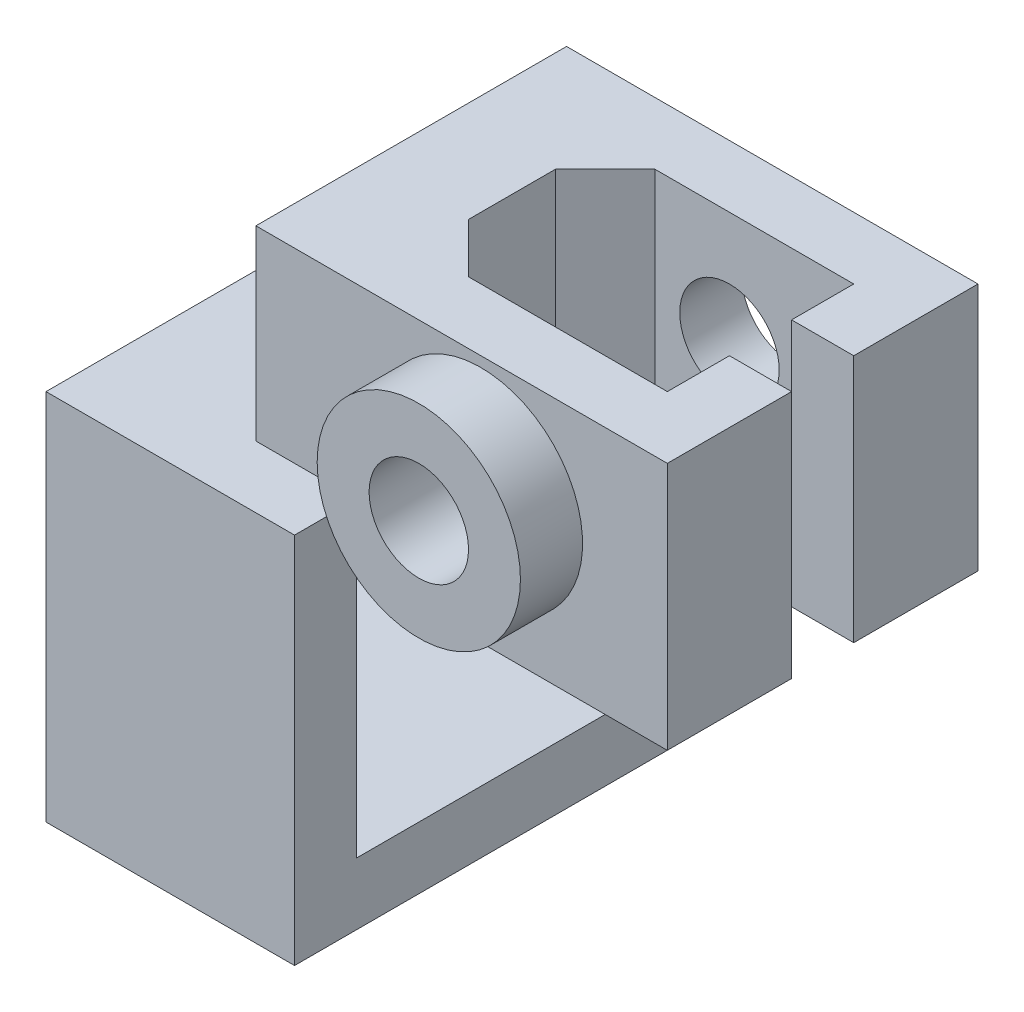
SolidWorks part; units mm, degrees
ref_plane "Front Plane" through (0, 0, 0) normal (0, 0, 1) x (1, 0, 0)
ref_plane "Top Plane" through (0, 0, 0) normal (0, 1, 0) x (1, 0, 0)
ref_plane "Right Plane" through (0, 0, 0) normal (1, 0, 0) x (0, 0, -1)
other "Configuration Table"
sketch "Sketch1" plane through (0, 0, 0) normal (0, 1, 0) x (1, 0, 0)
  line L1 (-20, 25) -> (20, 25)
  line L2 (-20, 25) -> (-20, -25)
  line L3 (-20, -25) -> (20, -25)
  line L4 (20, 25) -> (20, -25)
  line L5 (-20, 25) -> (20, -25) construction
  line L6 (-20, -25) -> (20, 25) construction
  point P0 (0, 0)
  dimension "D1" = 50
  dimension "D2" = 40
extrude "Boss-Extrude1" add sketch "Sketch1" along normal blind 10
sketch "Sketch2" plane through (0, 10, 0) normal (0, 1, 0) x (1, 0, 0)
  line L0 (28, -15) -> (60, -15)
  line L1 (20, -25) -> (20, 25) construction
  line L2 (60, -15) -> (60, -5)
  line L3 (60, -5) -> (70, -5)
  line L4 (70, -5) -> (70, -25)
  line L5 (70, -25) -> (20, -25)
  line L6 (20, -25) -> (20, -15)
  line L7 (20, 25) -> (70, 25)
  line L8 (70, 25) -> (70, 5)
  line L9 (70, 5) -> (60, 5)
  line L10 (60, 5) -> (60, 15)
  line L11 (60, 15) -> (28, 15)
  line L12 (20, 15) -> (20, 25)
  line L13 (28, 15) -> (20, 7)
  line L14 (28, -15) -> (20, -7)
  line L15 (20, -7) -> (20, -15)
  line L16 (20, 15) -> (20, 7)
  dimension "D1" = 50
  dimension "D2" = 40
  dimension "D3" = 10
  dimension "D4" = 50
  dimension "D5" = 40
  dimension "D6" = 10
  dimension "D7" = 8
  dimension "D8" = 8
  dimension "D9" = 10
  dimension "D10" = 8
  dimension "D11" = 8
  dimension "D12" = 10
extrude "Boss-Extrude2" add sketch "Sketch2" against normal blind 10
sketch "Sketch3" plane through (-20, 0, 0) normal (-1, 0, 0) x (0, 0, 1)
  line L0 (-25, 10) -> (-35, 10)
  line L1 (-35, 10) -> (-35, -50)
  line L2 (-35, -50) -> (35, -50)
  line L3 (35, -50) -> (35, 10)
  line L4 (35, 10) -> (25, 10)
  line L5 (25, 10) -> (25, 0)
  line L7 (-25, 0) -> (-25, 10)
  line L8 (-25, 0) -> (-25, -40)
  line L13 (-25, -40) -> (25, -40)
  line L14 (25, -40) -> (25, 0)
  line L15 (-25, 0) -> (25, 0) construction
  point P3 (0, -20.5094)
  dimension "D1" = 10
  dimension "D2" = 10
  dimension "D3" = 40
  dimension "D4" = 10
extrude "Boss-Extrude3" add sketch "Sketch3" against normal up to surface (40 mm away) up to face at (20, 5, 0)
sketch "Sketch4" plane through (0, 10, 0) normal (0, 1, 0) x (1, 0, 0)
  line L0 (20, 7) -> (28, 15)
  line L1 (28, 15) -> (60, 15)
  line L2 (60, 15) -> (60, 5)
  line L3 (60, 5) -> (70, 5) construction
  line L4 (60, 15) -> (60, 5) construction
  line L5 (60, 5) -> (70, 5)
  line L6 (70, 5) -> (70, 25)
  line L7 (70, 25) -> (3.7799, 25)
  line L8 (3.7799, 25) -> (3.7799, -25)
  line L9 (3.7799, -25) -> (70, -25)
  line L10 (70, -25) -> (70, -5)
  line L11 (70, -5) -> (60, -5)
  line L12 (60, -5) -> (60, -15)
  line L13 (60, -15) -> (28, -15)
  line L14 (28, -15) -> (20, -7)
  line L15 (20, -7) -> (20, 7)
extrude "Boss-Extrude4" add sketch "Sketch4" along normal blind 30
sketch "Sketch5" plane through (0, 0, -25) normal (0, 0, -1) x (-1, 0, 0)
  line L0 (-70, 0) -> (-20, 0) construction
  line L1 (-70, 0) -> (-70, 40) construction
  circle A0 centre (-40, 22) radius 8
  dimension "D1" = 16
  dimension "D2" = 22
  dimension "D3" = 30
extrude "Cut-Extrude1" cut sketch "Sketch5" against normal blind 50
sketch "Sketch6" plane through (0, 0, 25) normal (0, 0, 1) x (1, 0, 0)
  circle A0 centre (40, 22) radius 8
  circle A1 centre (40, 22) radius 16.3579
extrude "Boss-Extrude5" add sketch "Sketch6" along normal blind 10
